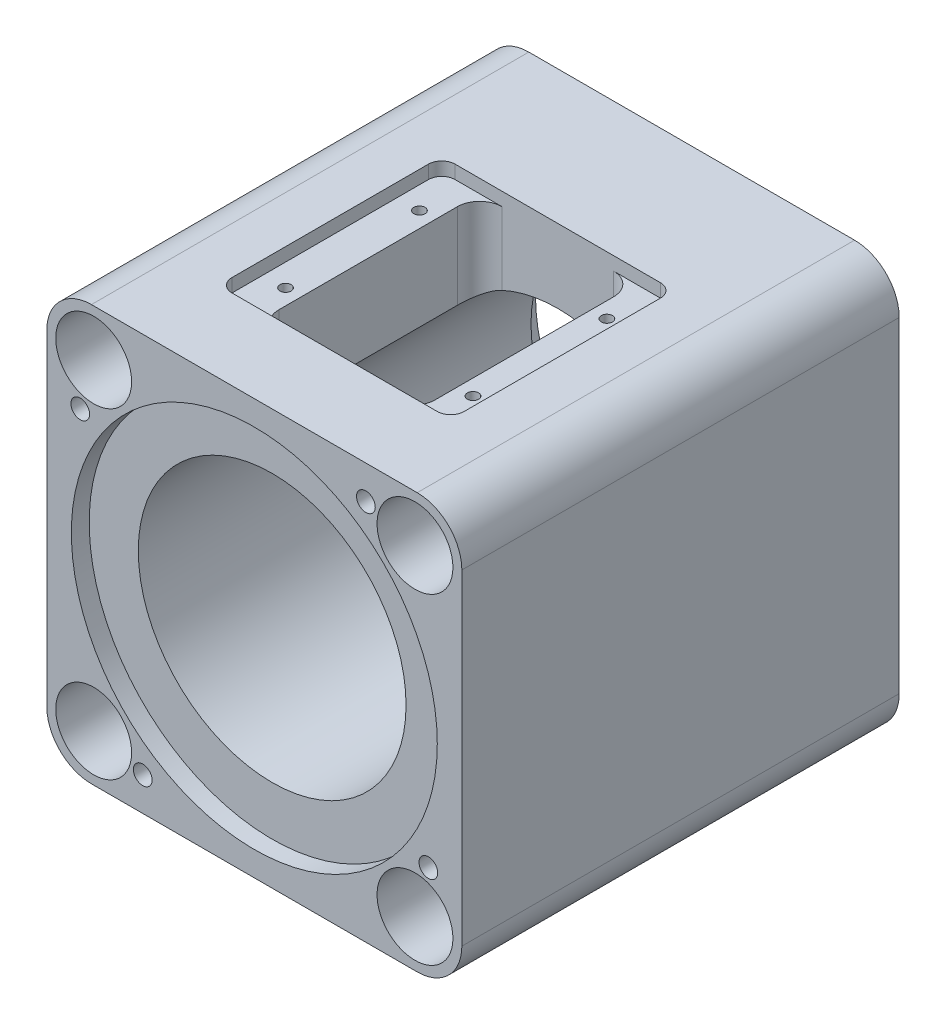
from build123d import *

# Parameters (mm, degrees)
SKETCH1_W                                = 93
SKETCH1_H                                = 93
BOSS_EXTRUDE1_DEPTH                      = 98
SKETCH2_R                                = 35
CUT_EXTRUDE1_DEPTH                       = 6
SKETCH3_R                                = 30
CUT_EXTRUDE2_DEPTH                       = 114.086250269
CUT_EXTRUDE3_REACH                       = 144.882
CUT_EXTRUDE3_END_RADIUS                  = 30
SKETCH4_W                                = 35
SKETCH4_H                                = 50
FILLET1_R                                = 10
CBORE_FOR_M10_HEX_HEAD_BOLT1_D           = 11
CBORE_FOR_M10_HEX_HEAD_BOLT1_CBORE_D     = 17
CBORE_FOR_M10_HEX_HEAD_BOLT1_CBORE_DEPTH = 78
SKETCH9_R                                = 41
CUT_EXTRUDE4_DEPTH                       = 4
SKETCH10_W                               = 52
SKETCH10_H                               = 50
CUT_EXTRUDE5_DEPTH                       = 3
FILLET2_R                                = 3
M3_TAPPED_HOLE1_D                        = 2.5
M3_TAPPED_HOLE1_DEPTH                    = 7.5
M3_TAPPED_HOLE1_TIP                      = 0.751075774
FILLET3_R                                = 5
CIRPATTERN1_COUNT                        = 4


with BuildPart() as part:
    # Sketch1 → Boss-Extrude1 (new body)
    with BuildSketch(Plane.XY):
        Rectangle(SKETCH1_W, SKETCH1_H)
    extrude(amount=BOSS_EXTRUDE1_DEPTH)

    # Sketch2 → Cut-Extrude1 (cut)
    with BuildSketch(Plane(origin=(0, 0, 0), x_dir=(-1, 0, 0), z_dir=(0, 0, -1))):
        Circle(SKETCH2_R)
    extrude(amount=-CUT_EXTRUDE1_DEPTH, mode=Mode.SUBTRACT)

    # Sketch3 → Cut-Extrude2 (cut, through all)
    with BuildSketch(Plane(origin=(0, 0, 6), x_dir=(-1, 0, 0), z_dir=(0, 0, -1))):
        Circle(SKETCH3_R)
    extrude(amount=-CUT_EXTRUDE2_DEPTH, mode=Mode.SUBTRACT)

    # Cut-Extrude3: up to this cylinder (the profile starts outside it)
    cut_extrude3_end = Plane(origin=(0, 0, 55), z_dir=(0, 0, -1)) * Cylinder(CUT_EXTRUDE3_END_RADIUS, 350.764, mode=Mode.PRIVATE)
    # Sketch4 → Cut-Extrude3 (cut, up to the surface)
    with BuildSketch(Plane(origin=(0, 46.5, 0), x_dir=(1, 0, 0), z_dir=(0, 1, 0)), mode=Mode.PRIVATE) as cut_extrude3_sk1:
        with Locations((0, -55)):
            Rectangle(SKETCH4_W, SKETCH4_H)
    cut_extrude3_tool1 = extrude(cut_extrude3_sk1.sketch, amount=-CUT_EXTRUDE3_REACH, mode=Mode.PRIVATE) - cut_extrude3_end
    add(cut_extrude3_tool1.solids().sort_by_distance((0, 46.5, 55))[0], mode=Mode.SUBTRACT)

    # Fillet1
    fillet1_edges = [part.edges().sort_by_distance(p)[0] for p in [
        (46.5, -46.5, 49),
        (-46.5, -46.5, 49),
        (-46.5, 46.5, 49),
        (46.5, 46.5, 49),
    ]]
    fillet(fillet1_edges, radius=FILLET1_R)

    # CBORE for M10 Hex Head Bolt1 (through all)
    with Locations(Plane.XY.offset(98)):
        with Locations((-36, 36), (36, 36), (36, -36), (-36, -36)):
            CounterBoreHole(CBORE_FOR_M10_HEX_HEAD_BOLT1_D / 2, CBORE_FOR_M10_HEX_HEAD_BOLT1_CBORE_D / 2, CBORE_FOR_M10_HEX_HEAD_BOLT1_CBORE_DEPTH)

    # Sketch9 → Cut-Extrude4 (cut)
    with BuildSketch(Plane.XY.offset(98)):
        Circle(SKETCH9_R)
    extrude(amount=-CUT_EXTRUDE4_DEPTH, mode=Mode.SUBTRACT)

    # Sketch10 → Cut-Extrude5 (cut)
    with BuildSketch(Plane(origin=(0, 46.5, 0), x_dir=(1, 0, 0), z_dir=(0, 1, 0))):
        with Locations((0, -55)):
            Rectangle(SKETCH10_W, SKETCH10_H)
    extrude(amount=-CUT_EXTRUDE5_DEPTH, mode=Mode.SUBTRACT)

    # Fillet2
    fillet2_edges = [part.edges().sort_by_distance(p)[0] for p in [
        (26, 45, 80),
        (-26, 45, 30),
        (26, 45, 30),
        (-26, 45, 80),
    ]]
    fillet(fillet2_edges, radius=FILLET2_R)

    # M3 Tapped Hole1
    with Locations(Plane(origin=(0, 43.5, 0), x_dir=(1, 0, 0), z_dir=(0, 1, 0))):
        with Locations((21, -40), (21, -70), (-21, -70), (-21, -40)):
            Hole(M3_TAPPED_HOLE1_D / 2, depth=M3_TAPPED_HOLE1_DEPTH)
            with Locations((0, 0, -(M3_TAPPED_HOLE1_DEPTH + M3_TAPPED_HOLE1_TIP / 2))):  # 118° drill point
                Cone(0, M3_TAPPED_HOLE1_D / 2, M3_TAPPED_HOLE1_TIP, mode=Mode.SUBTRACT)

    # Fillet3
    fillet3_edges = [part.edges().sort_by_distance(p)[0] for p in [
        (17.5, 33.933492931, 30),
        (17.5, 33.933492931, 80),
        (-17.5, 33.933492931, 80),
        (-17.5, 33.933492931, 30),
    ]]
    fillet(fillet3_edges, radius=FILLET3_R)

    # Sketch14 → M5 Tapped Hole2 (revolve, cut)
    with BuildSketch(Plane(origin=(25, 39, 98), x_dir=(0, -1, 0), z_dir=(1, 0, 0))):
        Polygon((0, 0), (0, 13.6618073), (2.1, 12.4), (2.1, 0), align=None)
    m5_tapped_hole2 = revolve(axis=Axis((25, 39, 104.35), (0, 0, -1)), mode=Mode.SUBTRACT)

    # CirPattern1: M5 Tapped Hole2 ×4 about axis
    cirpattern1_axis = Axis((0, 0, 0), (0, 0, 1))
    for i in range(1, CIRPATTERN1_COUNT):
        add(m5_tapped_hole2.rotate(cirpattern1_axis, i * 360 / CIRPATTERN1_COUNT), mode=Mode.SUBTRACT)


solid = part.part
